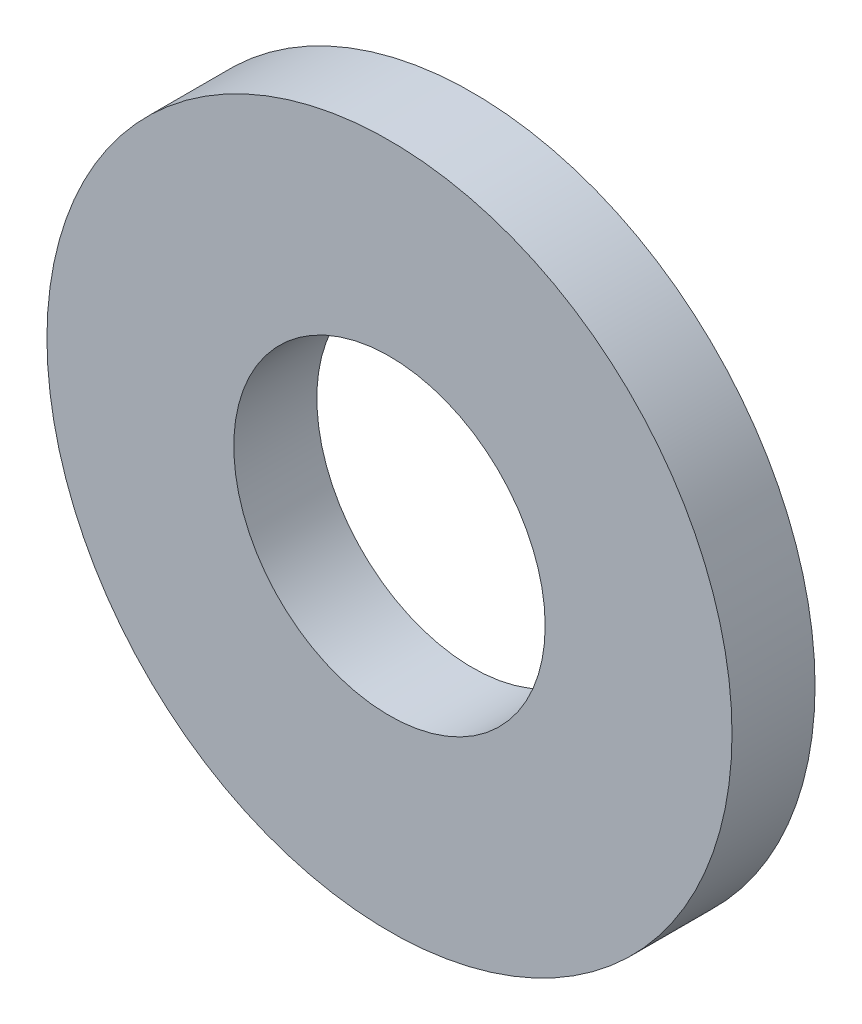
SolidWorks part; units mm, degrees
ref_plane "Front Plane" through (0, 0, 0) normal (0, 0, 1) x (1, 0, 0)
ref_plane "Top Plane" through (0, 0, 0) normal (0, 1, 0) x (1, 0, 0)
ref_plane "Right Plane" through (0, 0, 0) normal (1, 0, 0) x (0, 0, -1)
sketch "Sketch1" plane through (0, 0, 0) normal (0, 0, 1) x (1, 0, 0)
  circle A0 centre (0, 0) radius 82.5
  circle A1 centre (0, 0) radius 37.5
  dimension "D1" = 165
  dimension "D2" = 75
extrude "Boss-Extrude1" add sketch "Sketch1" along normal blind 20
